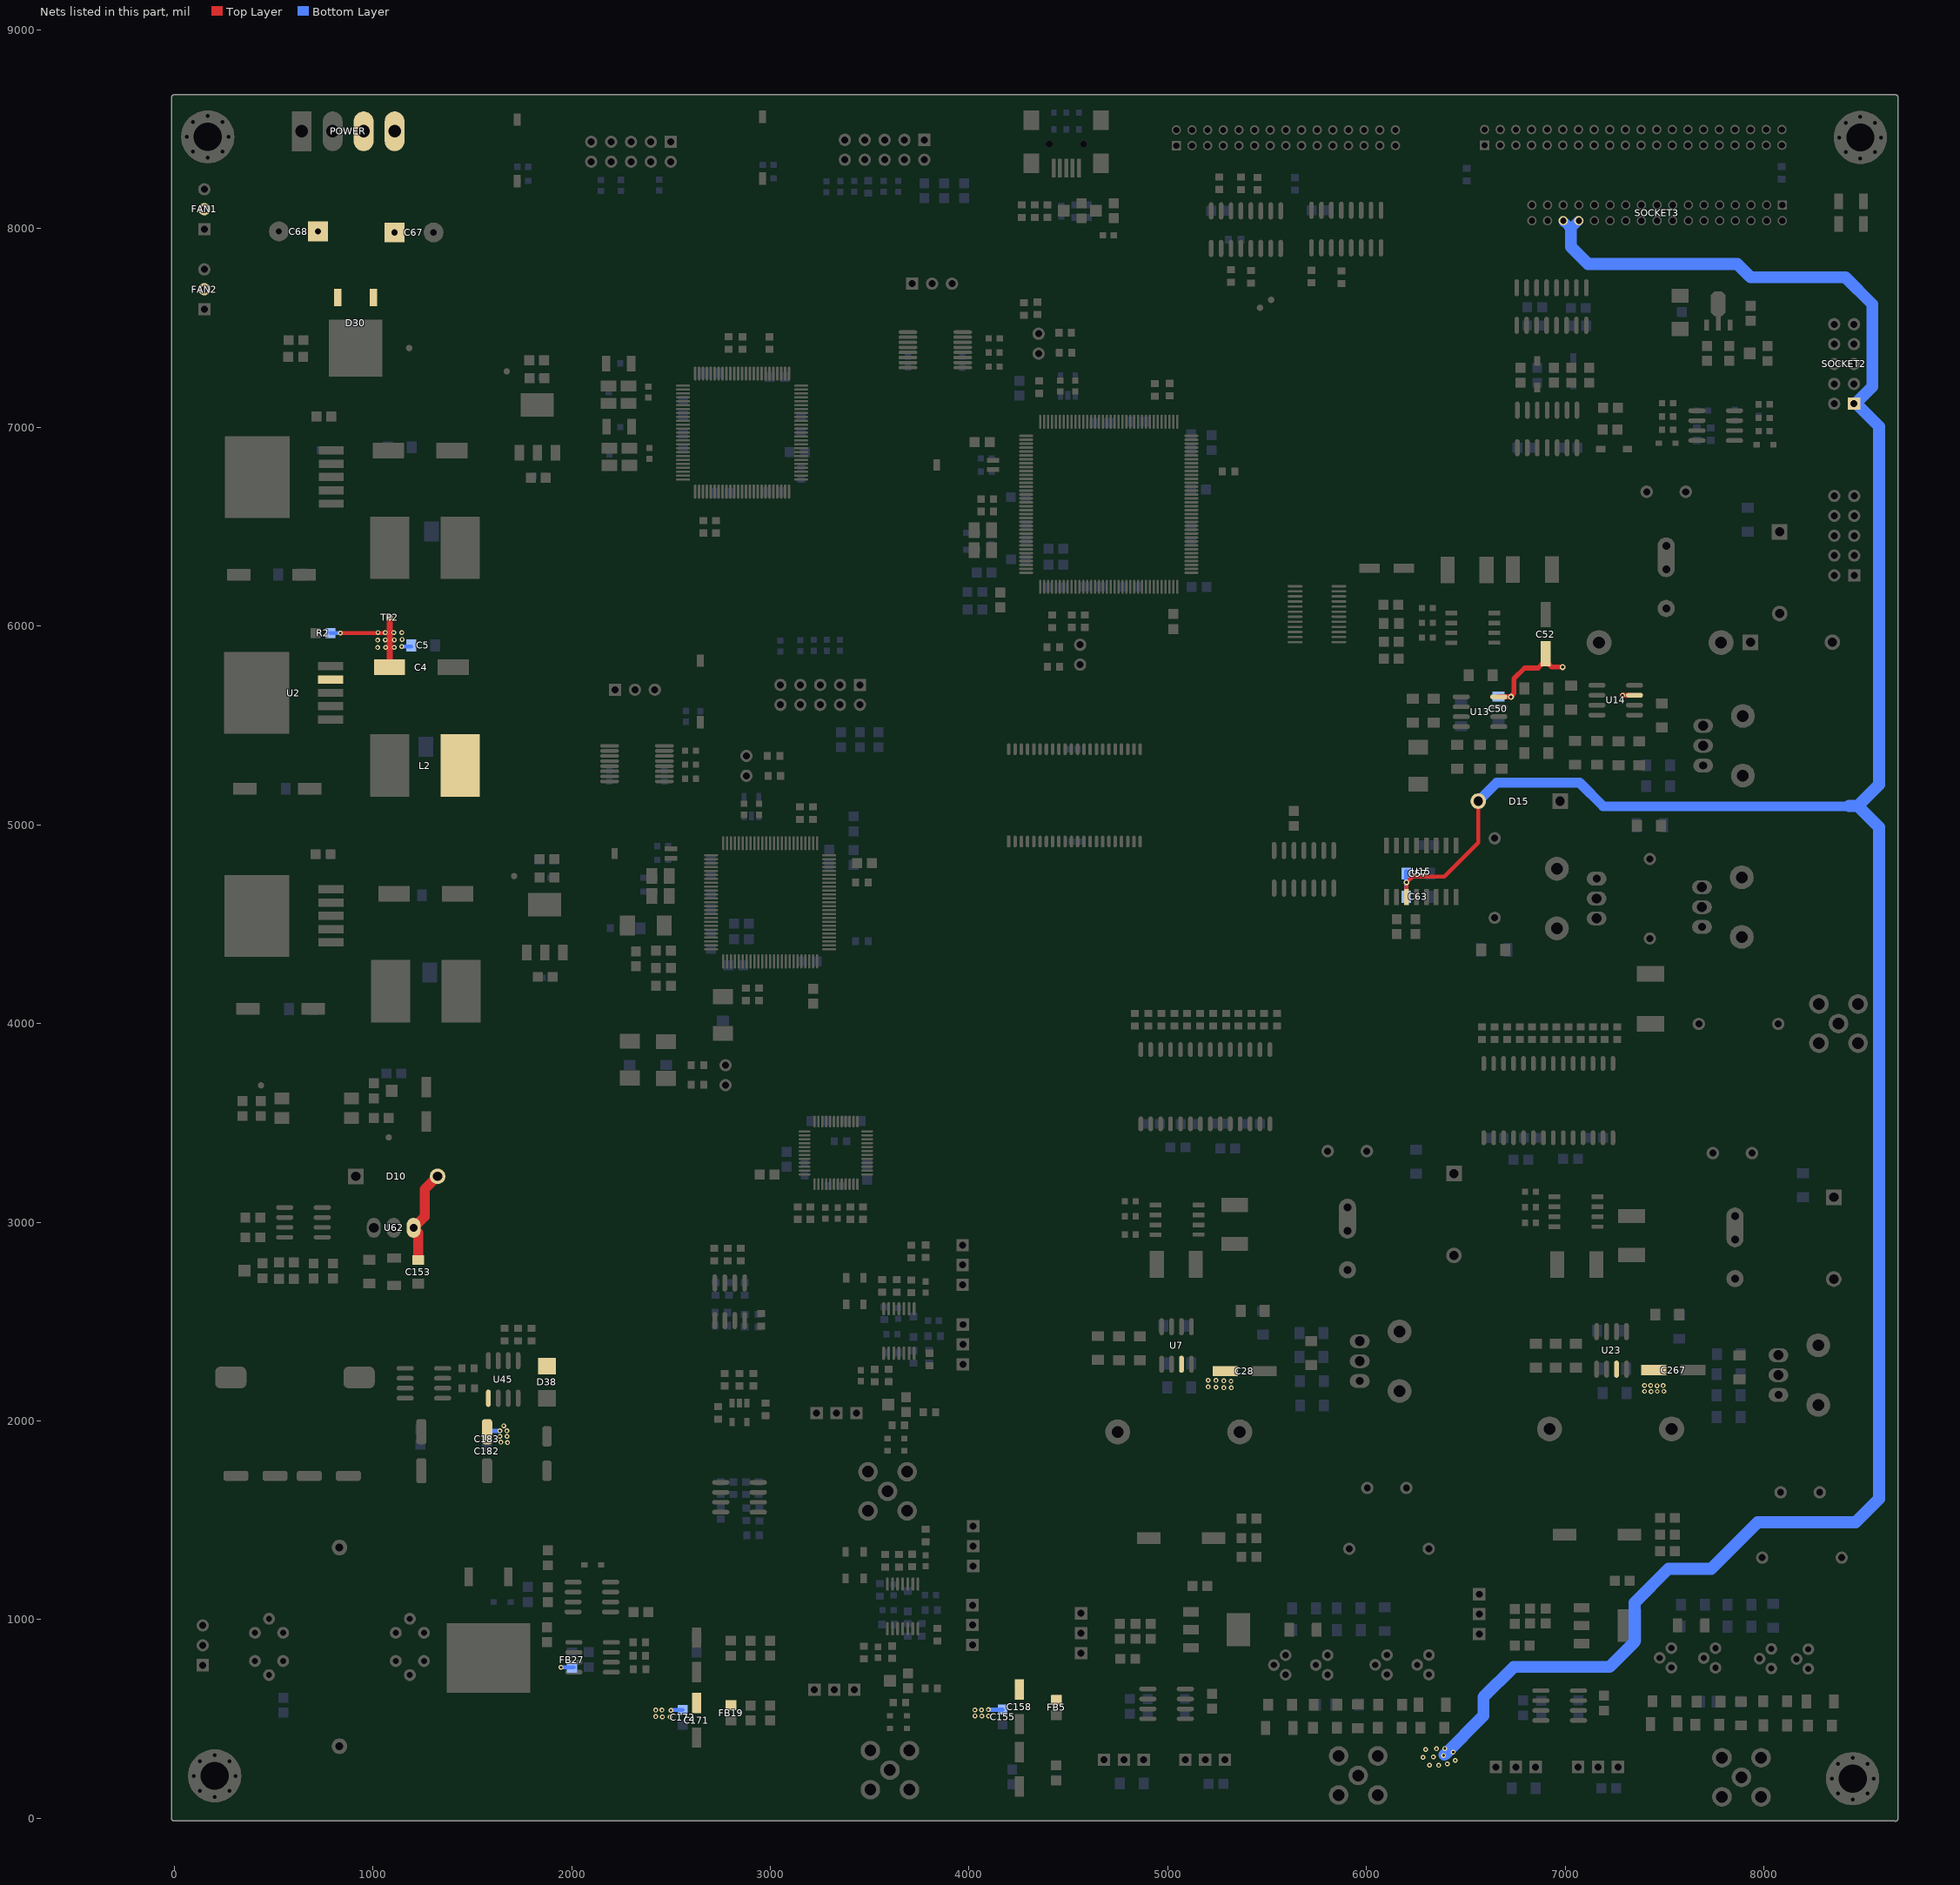
[diagram p0: the nets of this part, all layers, seen from the top]
# Altium PCB MISC82309.PcbDoc (part 4 of 14)
Units mil, origin at the board's own origin, x right, y up, seen from the top; angles counter-clockwise.
Board outline 8687.03 x 8687.86 mil, 4 copper layers (Top Layer, GND, POWER, Bottom Layer); 747 components, 583 nets, 2530 pads, 1834 vias.

## Footprints (in the part's own frame and the unit in brackets; to place one, negate y for a bottom-side part, rotate by r counter-clockwise, add the part's x,y. Pads: shape width x height; smd on the part's side, far side on the other; paste and mask are expansions set on the pad) (continued)
P-DSO-8 [mm]
  rect 1.5x0.6 smd: 1(0,0) 2(0,-1.27) 3(0,-2.54) 4(0,-3.81) 6(5.5,-2.54) 7(5.5,-1.27) 8(5.5,0)
  rect 1.5x0.5 smd: 5(5.5,-3.81)
  silkscreen extent 0.95,-4.51 4.55,0.7
PBS5022 [mm]
  rrect50% 4x2.79 smd: 1(-8.2,0) 2(8.2,0)
  silkscreen extent -9.27,-7.62 9.27,7.62, body extent -9.02,-7.37 9.02,7.37, height 7.51
PLS-2-2_54 [mil] "ZL201 SERIES 2.54 MM (0.100'') STRAIGHT PIN HEADER"
  round 62 hole 35: 1(0,0) 2(100,0)
  silkscreen extent -50,-50 150,50, body extent -50,-50 150,50, height 336
R0603 [mm]
  rect 0.8x0.8 smd: 1(-0.698,0) 2(0.698,0)
  silkscreen extent -1.46,-0.7 1.46,0.7, body extent -0.8,-0.4 0.8,0.4, height 0.4
R0805 [mil]
  rect 50x50 smd: 1(-37.5,0) 2(37.5,0)
  silkscreen extent -80,-38 80,38
R1206 [mil]
  rect 50x60 smd: 1(-60,0) 2(60,0)
  silkscreen extent -94,-41 94,41, body extent -63,-31 63,31, height 22
Radj [mil]
  rect 62x62 hole 35: 1(0,0) 2(100,0) 3(200,0)
  silkscreen extent -90,-110 290,103, body extent -88,-95 288,95, height 455
RES_0603 [mm]
  rect 0.9x1 smd: 1(-0.8,0) 2(0.8,0)
  silkscreen extent -1.45,-0.7 1.45,0.7, body extent -0.8,-0.4 0.8,0.41, height 0.4
RES_0805 [mil]
  rect 50x50 smd: 1(-37.5,0) 2(37.5,0)
  silkscreen extent -70,-32 70,32, body extent -39,-25 39,25, height 20
RES_2512 [mm]
  rect 2x3.5 smd: 1(-3.2,0) 2(3.2,0)
  silkscreen extent -4.45,-2.03 4.45,2.03, body extent -3.2,-1.6 3.2,1.6, height 0.6
RM8 [mil]
  round 60 hole 30: 1(-425.2,70.87) 2(-425.2,-70.87) 3(-354.33,141.73) 4(-354.33,-141.73) 5(-283.46,70.87) 6(-283.46,-70.87) 7(425.2,70.87) 8(425.2,-70.87) 9(354.33,141.73) 10(354.33,-141.73) 11(283.46,70.87) 12(283.46,-70.87)
  round 78.74 hole 39.37: M-1(0,500) M-2(0,-500)
  silkscreen extent -462,-329 462,329, body extent -466,-502 466,502, height 642
SB560 [mm]
  round 3.2 hole 1.524: 1(0,0) 2(15.6,0)
  silkscreen extent 2.54,-2.54 12.95,2.54, body extent -0.7,-2.79 16.2,2.85, height 5.82
SMB_V-RJ45#1 [mm] "Connector; SMB Straight"
  round 2.5 hole 1.5: 1(0,0) 2(-2.5,-2.5) 2(-2.5,2.5) 2(2.5,-2.5) 2(2.5,2.5)
  silkscreen extent -3.15,-3.15 3.15,3.15
SMB_V-RJ45#2 [mm] "Connector; SMB Straight"
  round 2.5 hole 1.5: 1(0,0) M-1(-2.5,2.5) M-2(2.5,2.5) M-3(2.5,-2.5) M-4(-2.5,-2.5)
  silkscreen extent -3.15,-3.15 3.15,3.15, body extent -3.5,-3.5 3.5,3.5, height 7.56
SMD0805-L [mm] "Molded Inductor, 2-Leads, Body 2.00x1.25mm, IPC Medium Density"
  rect 1.25x1.35 smd: 1(-0.975,0) 2(0.975,0)
  silkscreen extent -1.85,-0.94 1.85,0.94, body extent -1.1,-0.7 1.1,0.7, height 0.6
SMD1206-L [mm] "Chip Inductor, 2-Leads, Body 3.25x1.65mm, IPC Medium Density"
  rect 1.1x2 smd: 1(-1.6,0) 2(1.6,0)
  silkscreen extent -2.45,-1.26 2.45,1.24, body extent -1.75,-0.9 1.75,0.9, height 1.27
SMD1812-Fuse [mm] "Chip Fuse, 2-Leads, Body 4.55x3.24mm, IPC Medium Density"
  rect 1.8x3.4 smd: 1(-2.49,0) 2(2.49,0)
  silkscreen extent -3.68,-1.98 3.71,2.01, body extent -2.25,-1.6 2.25,1.6, height 0.38
SMD5032 [mm]
  rect 2x1.4 smd: 1(0,0) 2(2.54,0) 3(2.54,2.2) 4(0,2.2)
  silkscreen extent -1.22,-1.37 3.78,3.12
SO8 [mm] "SOIC, 8-Leads, Body 4.9x3.9mm, Pitch 1.27mm, IPC Medium Density"
  oval 2.2x0.6 smd: 1(-2.4,1.905) 2(-2.4,0.635) 3(-2.4,-0.635) 4(-2.4,-1.905) 5(2.4,-1.905) 6(2.4,-0.635) 7(2.4,0.635) 8(2.4,1.905)
  silkscreen extent -2.52,-2.5 0.9,2.88, body extent -3,-2.45 3,2.45, height 1.7
SO8_N [mm] "SOIC, 8-Leads, Body 4.9x3.9mm, Pitch 1.27mm, IPC Medium Density"
  oval 2.2x0.6 smd: 1(-2.4,1.905) 2(-2.4,0.635) 3(-2.4,-0.635) 4(-2.4,-1.905) 5(2.4,-1.905) 6(2.4,-0.635) 7(2.4,0.635) 8(2.4,1.905)
  silkscreen extent -2.53,-2.5 0.9,2.88, body extent -1.95,-2.45 1.95,2.45, height 1.75
SO14 [mm] "SOIC, 14-Leads, Body 8.7x3.9mm, Pitch 1.27mm, IPC Medium Density"
  oval 2.2x0.6 smd: 1(-2.4,3.81) 2(-2.4,2.54) 3(-2.4,1.27) 4(-2.4,0) 5(-2.4,-1.27) 6(-2.4,-2.54) 7(-2.4,-3.81) 8(2.4,-3.81) 9(2.4,-2.54) 10(2.4,-1.27) 11(2.4,0) 12(2.4,1.27) 13(2.4,2.54) 14(2.4,3.81)
  silkscreen extent -2.52,-4.4 0.9,4.78, body extent -3.07,-4.35 3.07,4.35, height 1.78
SO14_N [mm] "SOIC, 14-Leads, Body 8.7x3.9mm, Pitch 1.27mm, IPC Medium Density"
  oval 2.2x0.6 smd: 1(-2.4,3.81) 2(-2.4,2.54) 3(-2.4,1.27) 4(-2.4,0) 5(-2.4,-1.27) 6(-2.4,-2.54) 7(-2.4,-3.81) 8(2.4,-3.81) 9(2.4,-2.54) 10(2.4,-1.27) 11(2.4,0) 12(2.4,1.27) 13(2.4,2.54) 14(2.4,3.81)
  silkscreen extent -2.52,-4.4 0.9,4.79, body extent -1.95,-4.33 1.95,4.33, height 1.75
SO-8_N [mm] "SOIC, 8-Leads, Body 4.9x3.9mm, Pitch 1.27mm, IPC Medium Density"
  oval 2.2x0.6 smd: 1(-2.4,1.905) 2(-2.4,0.635) 3(-2.4,-0.635) 4(-2.4,-1.905) 5(2.4,-1.905) 6(2.4,-0.635) 7(2.4,0.635) 8(2.4,1.905)
  silkscreen extent -2.52,-2.5 0.9,2.88, body extent -2,-2.5 2,2.5, height 1.75
SOD323 [mm]
  rect 0.8x0.7 smd: 1(1.075,0) 2(-1.075,0)
  silkscreen extent -0.66,-0.68 0.66,0.68, body extent -1.35,-0.62 1.35,0.63, height 1.1
SOD-123 [mm] "SOD-123; 2 Leads; Body 2.7 x 1.6 mm, (LxW)"
  rect 1.2x0.8 smd: 1(-1.7,0) 2(1.7,0)
  silkscreen extent -0.89,-0.8 0.89,0.81, body extent -1.85,-0.8 1.85,0.8, height 1.25
SOD-323 [mm]
  rect 1x1 smd paste+0.02 mask+0.05: 1(0,0) 2(0,2.6)
  silkscreen extent -0.68,0.64 0.68,1.95, body extent -0.68,-0.26 0.68,2.86, height 1
SOIC-8 [mm] "SOIC, 8-Leads, Body 4.9x3.9mm, Pitch 1.27mm, IPC Medium Density"
  oval 2.2x0.6 smd: 1(-2.4,1.905) 2(-2.4,0.635) 3(-2.4,-0.635) 4(-2.4,-1.905) 5(2.4,-1.905) 6(2.4,-0.635) 7(2.4,0.635) 8(2.4,1.905)
  silkscreen extent -2.52,-2.5 0.9,2.88, body extent -3,-2.45 3,2.45, height 1.7
SOIC-16 [mil]
  rect 80x24 smd: 1(-130,175) 2(-130,125) 3(-130,75) 4(-130,25) 5(-130,-25) 6(-130,-75) 7(-130,-125) 8(-130,-175) 9(130,-175) 10(130,-125) 11(130,-75) 12(130,-25) 13(130,25) 14(130,75) 15(130,125) 16(130,175)
  silkscreen extent -209,-205 77,205
SOIC_4N [mm] "SOT143, 4-Leads, Body 4.77x9.80mm, Pitch 2.55mm, IPC Medium Density"
  rect 1.9x1.5 smd: 1(-4.45,1.275) 2(-4.45,-1.275) 3(4.45,-1.275) 4(4.45,1.275)
  silkscreen extent -4.58,-2.5 3.5,2.7, body extent -5,-2.47 5,2.48, height 3.83
SOIC_8N [mm] "SOIC, 8-Leads, Body 4.90x3.90mm, Pitch 1.27mm, IPC Medium Density"
  oval 2.2x0.6 smd: 1(-2.4,1.905) 2(-2.4,0.635) 3(-2.4,-0.635) 4(-2.4,-1.905) 5(2.4,-1.905) 6(2.4,-0.635) 7(2.4,0.635) 8(2.4,1.905)
  silkscreen extent -2.52,-2.5 0.9,2.88, body extent -3.1,-2.5 3.1,2.5, height 1.75
SOP127P1020X265-28N [mm] "SOP, 28-Leads, Body 17.90x7.50mm, Pitch 1.27mm, IPC Medium Density"
  oval 1.9x0.6 smd: 1(-4.75,8.255) 2(-4.75,6.985) 3(-4.75,5.715) 4(-4.75,4.445) 5(-4.75,3.175) 6(-4.75,1.905) 7(-4.75,0.635) 8(-4.75,-0.635) 9(-4.75,-1.905) 10(-4.75,-3.175) 11(-4.75,-4.445) 12(-4.75,-5.715) 13(-4.75,-6.985) 14(-4.75,-8.255) 15(4.75,-8.255) 16(4.75,-6.985) 17(4.75,-5.715) 18(4.75,-4.445) 19(4.75,-3.175) 20(4.75,-1.905) 21(4.75,-0.635) 22(4.75,0.635) 23(4.75,1.905) 24(4.75,3.175) 25(4.75,4.445) 26(4.75,5.715) 27(4.75,6.985) 28(4.75,8.255)
  silkscreen extent -4.87,-9.05 3.4,9.23, body extent -5.26,-9.04 5.41,9.04, height 2.39
SOT23-5_M [mm]
  rect 1.1x0.65 smd: 1(1.2,-0.95) 2(1.2,0) 3(1.2,0.95) 4(-1.2,0.95) 5(-1.2,-0.95)
  silkscreen extent -0.25,-1.95 1.32,1.5, body extent -0.87,-1.5 0.88,1.5, height 1.45
SOT89 [mm]
  rect 1.4x0.6 smd: 1(-1.673,1.5) 3(-1.673,-1.5)
  rect 1.8x0.6 smd: 2(-1.473,0)
  oct 3.2x1.9 smd: 2(1.027,0)
  silkscreen extent -1.95,-2.3 1.43,2.47, body extent -2.31,-2.31 1.94,2.29, height 1.6
SOT223 [mm]
  rect 2x1.2 smd: 1(0,0.014) 2(0,-2.286) 3(0,-4.586)
  rect 3x4.2 smd: 4(6.096,-2.272)
  silkscreen extent 1.27,-5.7 4.32,1.28, body extent -0.3,-5.51 6.7,0.99, height 1.7
SOT-23 [mil]
  rect 50x50 smd: 1(0,0) 2(0,-75)
  rect 60x60 smd: 3(90,-38)
  silkscreen extent 5,-95 95,20, body extent -5,-97 95,21, height 43
SOT-23-3 [mil]
  rect 50x50 smd: 1(-45,37.5) 2(-45,-37.5)
  rect 60x60 smd: 3(45,-0.5)
  silkscreen extent -40,-58 50,58, body extent -50,-60 50,59, height 43
SSOP16_M [mm] "SOP, 16-Leads, Body 6.2x5.3mm, Pitch 0.65mm, IPC Low Density"
  oval 2.4x0.45 smd: 1(-3.5,2.275) 2(-3.5,1.625) 3(-3.5,0.975) 4(-3.5,0.325) 5(-3.5,-0.325) 6(-3.5,-0.975) 7(-3.5,-1.625) 8(-3.5,-2.275) 9(3.5,-2.275) 10(3.5,-1.625) 11(3.5,-0.975) 12(3.5,-0.325) 13(3.5,0.325) 14(3.5,0.975) 15(3.5,1.625) 16(3.5,2.275)
  silkscreen extent -3.63,-3.25 1.9,3.25, body extent -3.81,-3.25 3.81,3.25, height 1.99
SW-6X3X2.5 [mil] "Switch, 6x3x2.5mm"
  rect 62.99x35 smd: 1(-155,0) 2(155,0)
  silkscreen extent -118,-69 118,69, body extent -157,-73 157,73, height 98
TO220 [mil]
  oval 100x70 hole 50: 1(0,100) 2(0,0)
  oval 100x70 hole 40: 3(0,-100)
  silkscreen extent -69,-200 131,200, body extent -55,-200 125,200, height 723
TO220V1 [mil]
  oval 100x70 hole 50: 1(0,100) 2(0,0)
  oval 100x70 hole 40: 3(0,-100)
  round 120 hole 59: M-1(200,150) M-2(200,-150)
  silkscreen extent -100,-383 321,384, body extent -55,-374 311,374, height 986
TO-92 [mm]
  round 1.5 hole 0.8: 1(0,-1.25) 2(-1.5,0) 3(0,1.25)
  silkscreen extent -2.66,-2.66 1.91,2.66, body extent -2.64,-2.67 1.52,2.65, height 8.33
TO-252AA [mm] "D-PAK, 3-Pads, Body 6.21x6.73mm (max), IPC Medium Density"
  rect 2.25x0.95 smd: 1(-4.45,2.28) 3(-4.45,-2.28)
  rect 7.3x6.8 smd: 4(2,0)
  silkscreen extent -4.57,-3.35 -2.05,3.43, body extent -4.7,-3.3 5,3.28, height 2.3
TPOINT [mil]
  round 32 smd: 1(0,0)
  silkscreen extent -25,-25 25,25
TQFP100_N [mm]
  oval 0.3x1.8 smd: 1(-6,-7.55) 2(-5.5,-7.55) 3(-5,-7.55) 4(-4.5,-7.55) 5(-4,-7.55) 6(-3.5,-7.55) 7(-3,-7.55) 8(-2.5,-7.55) 9(-2,-7.55) 10(-1.5,-7.55) 11(-1,-7.55) 12(-0.5,-7.55) 13(0,-7.55) 14(0.5,-7.55) 15(1,-7.55) 16(1.5,-7.55) 17(2,-7.55) 18(2.5,-7.55) 19(3,-7.55) 20(3.5,-7.55) 21(4,-7.55) 22(4.5,-7.55) 23(5,-7.55) 24(5.5,-7.55) 25(6,-7.55) 51(6,7.55) 52(5.5,7.55) 53(5,7.55) 54(4.5,7.55) 55(4,7.55) 56(3.5,7.55) 57(3,7.55) 58(2.5,7.55) 59(2,7.55) 60(1.5,7.55) 61(1,7.55) 62(0.5,7.55) 63(0,7.55) 64(-0.5,7.55) 65(-1,7.55) 66(-1.5,7.55) 67(-2,7.55) 68(-2.5,7.55) 69(-3,7.55) 70(-3.5,7.55) 71(-4,7.55) 72(-4.5,7.55) 73(-5,7.55) 74(-5.5,7.55) 75(-6,7.55)
  oval 1.8x0.3 smd: 26(7.55,-6) 27(7.55,-5.5) 28(7.55,-5) 29(7.55,-4.5) 30(7.55,-4) 31(7.55,-3.5) 32(7.55,-3) 33(7.55,-2.5) 34(7.55,-2) 35(7.55,-1.5) 36(7.55,-1) 37(7.55,-0.5) 38(7.55,0) 39(7.55,0.5) 40(7.55,1) 41(7.55,1.5) 42(7.55,2) 43(7.55,2.5) 44(7.55,3) 45(7.55,3.5) 46(7.55,4) 47(7.55,4.5) 48(7.55,5) 49(7.55,5.5) 50(7.55,6) 76(-7.55,6) 77(-7.55,5.5) 78(-7.55,5) 79(-7.55,4.5) 80(-7.55,4) 81(-7.55,3.5) 82(-7.55,3) 83(-7.55,2.5) 84(-7.55,2) 85(-7.55,1.5) 86(-7.55,1) 87(-7.55,0.5) 88(-7.55,0) 89(-7.55,-0.5) 90(-7.55,-1) 91(-7.55,-1.5) 92(-7.55,-2) 93(-7.55,-2.5) 94(-7.55,-3) 95(-7.55,-3.5) 96(-7.55,-4) 97(-7.55,-4.5) 98(-7.55,-5) 99(-7.55,-5.5) 100(-7.55,-6)
  silkscreen extent -6.82,-7.67 6.25,6.25, body extent -7,-7 7,7, height 1.6
TS5B_N [mm] "D2-PAK, 6-Leads, Body 8.6x10.2mm, Pitch 1.7mm, Lead Span 14.1mm, IPC Medium Density"
  rect 3.2x1.05 smd: 1(-6,3.4) 2(-6,1.7) 3(-6,0) 4(-6,-1.7) 5(-6,-3.4)
  rect 8.3x10.45 smd: 6(3.45,0)
  silkscreen extent -6.13,-5.2 -1.1,5.2, body extent -2.65,-5.2 6.24,5.2, height 4.65
TSOP44-IS61LV51216AL-10TLI [mm] "512K x 16 HIGH SPEED ASYNCHRONOUS  CMOS STATIC RAM WITH 3.3V SUPPLY"
  rect 1.5x0.45 smd: 1(0,0)
  oval 1.5x0.45 smd: 2(0,-0.8) 3(0,-1.6) 4(0,-2.4) 5(0,-3.2) 6(0,-4) 7(0,-4.8) 8(0,-5.6) 9(0,-6.4) 10(0,-7.2) 11(0,-8) 12(0,-8.8) 13(0,-9.6) 14(0,-10.4) 15(0,-11.2) 16(0,-12) 17(0,-12.8) 18(0,-13.6) 19(0,-14.4) 20(0,-15.2) 21(0,-16) 22(0,-16.8) 23(11.8,-16.8) 24(11.8,-16) 25(11.8,-15.2) 26(11.8,-14.4) 27(11.8,-13.6) 28(11.8,-12.8) 29(11.8,-12) 30(11.8,-11.2) 31(11.8,-10.4) 32(11.8,-9.6) 33(11.8,-8.8) 34(11.8,-8) 35(11.8,-7.2) 36(11.8,-6.4) 37(11.8,-5.6) 38(11.8,-4.8) 39(11.8,-4) 40(11.8,-3.2) 41(11.8,-2.4) 42(11.8,-1.6) 43(11.8,-0.8) 44(11.8,0)
  silkscreen extent 1.58,-17.2 10.3,0.4, body extent 0.03,-17.54 11.79,0.67, height 1.3
TSSOP-24 [mm]
  oval 1.9x0.3 smd: 1(-2.8,3.575) 2(-2.8,2.925) 3(-2.8,2.275) 4(-2.8,1.625) 5(-2.8,0.975) 6(-2.8,0.325) 7(-2.8,-0.325) 8(-2.8,-0.975) 9(-2.8,-1.625) 10(-2.8,-2.275) 11(-2.8,-2.925) 12(-2.8,-3.575) 13(2.8,-3.575) 14(2.8,-2.925) 15(2.8,-2.275) 16(2.8,-1.625) 17(2.8,-0.975) 18(2.8,-0.325) 19(2.8,0.325) 20(2.8,0.975) 21(2.8,1.625) 22(2.8,2.275) 23(2.8,2.925) 24(2.8,3.575)
  silkscreen extent -1.6,-4 1.6,4
U5+1_N [mm] "SOT23, 5-Leads, Body 2.9x1.6mm, Pitch 0.95mm, Lead Span 2.8mm, IPC Medium Density"
  rect 1.1x0.65 smd: 1(-1.2,0.95) 2(-1.2,0) 3(-1.2,-0.95) 4(1.2,-0.95) 5(1.2,0.95)
  silkscreen extent -1.32,-1.5 0.25,1.95, body extent -0.87,-1.5 0.87,1.5, height 1.45
VH-3_96-4 [mm]
  rect 2.54x5.08 hole 1.6: 1(0,0)
  oval 2.54x5.08 hole 1.6: 2(3.96,0) 3(7.92,0) 4(11.88,0)
  silkscreen extent -1.98,-4.8 13.86,3.7, body extent -1.95,-4.8 13.83,3.7, height 10.73
Y_XTAL_T7 [mm]
  rect 0.6x1.6 smd: 1(1.235,0.254) 4(0.035,0.254)
  rect 0x0 smd: 2(0.635,6.858)
  rect 1.4x0.8 smd: 3(0.635,7.454)
  silkscreen extent -0.17,0.25 1.44,7.25, body extent -0.24,-0.38 1.51,7.56, height 1.6

## Part data
C1 C2 C6 C7 C8 C14 C16 C18 C19 C20 C34 C39 C40 C41 C65 C66 C74 C75 C79 C80 C81 C84 C85 C86 C87 C88 C89 C98 C99 C123 C124 C125 C126 C127 C128 C129 C130 C131 C132 C133 C134 C141 C142 C143 C146 C147 C148 C172 C173 C175 C176 C193 C195 C196 C197 C198 C199 C200 C201 C202 C242 C243 C244 C245 C246 C247 C248 C249 C250 C251 C252 C253 C254 C255 C449: library part CAP_1206, "Capacitor"
C3 C4 C9 C10 C11 C12: library part "CAP POL"
C5 C13 C15 C42 C155 C156 C280 C281: library part CAP_0.1uF
C17 C64 C158 C159 C171 C174: library part CAP_POLAR_1, "Polar Capacitor"
C23 C47 C265: library part CAP_47pF, "Capacitor 47pF"
C24 C49 C270: library part CAP_10nF, "Capacitor 10nF"
C25 C48 C271: library part CAP_2.2nF, "Capacitor 2.2nF"
C27 C51 C263: library part CAP_470pF, "Capacitor 470pF"
C28 C52 C267: library part CAP_POLAR_22uF_35V, "Polar Capacitor 22uF 35V"
C29 C54 C266: library part CAP_POLAR_2.2uF_450V, "Polar Capacitor 222uF 450V"
C30 C31 C32 C33 C56 C63 C153 C157 C277 C282 C283 C284 C285 C317 C318: library part CAP_0.1uF, "Capacitor 0.1uF"
C35 C36 C37 C38 C70 C71 C72 C73 C82 C83 C151 C154 C162 C183 C184 C214 C215 C220 C221 C231 C233 C256 C257 C373 C374: library part CAP_0805, "Capacitor"
C45: library part CAP_0.22uF, "Capacitor 0.22uF"
C50 C53 C69 C278: library part CAP_0.47uF, "Capacitor 0.47uF"
C55 C188 C279: library part CAP_CBB_0.33uF_400V, "CBB Capacitor 0.33uF 400V"
C57: library part CAP_AVX_4.7uF_16V, "AVX Capacitor 4.7uFF 16V"
C58: library part CAP_CBB_0.1uF_400V, "CBB Capacitor0.1uF 400V"
C62: library part CAP_CBB_22nF_630V, "CBB Capacitor 22nF 630V"
C67 C68: library part CAP_EL, "Capacitor"
C78: library part CAP_0.1uF, "Capacitor 0.33uF"
C90 C91 C92 C93 C94 C177 C178 C179 C180 C181: library part CAP_0402, "Capacitor"
C163 C164 C363 C364: library part Cap, "Capacitor"
C165 C166 C167 C168 C169 C170 C210 C226 C232 C240 C241 C288 C289 C290 C291 C292 C293 C311 C330 C370 C411 C412 C413 C420 C421 C422 C423 C424 C501 C502 C599: library part CAP_0603, "Capacitor"
C182 C227 C228 C229 C230: library part CAP_ALU, "Capacitor"
C187 C276: library part CAP_0.22nF, "Capacitor 0.22nF"
C506 C507: "Capacitor (Semiconductor SIM Model)"
CH-DET_A CH-DET_B CHARGE-OUT_A CHARGE-OUT_B MOD-OUT: "SMB Straight Connector"
CPLD-JTAG D-JTAG P-JTAG SOCKET1 SOCKET2: library part HEAD2X5-2_54
D10: library part UF400X
D23 D28 D29 D34: "1SMA4728A 1W 3.3V SMA DO-214AC"
D24 D52 D54: library part BZT52C4V7
D27 D48: library part Diode-SMD
D40: library part UF4007
D55: library part 1N4001/M1
ESD23 ESD24 ESD25: library part DIODE_TVS_BI-DIR, "TVS,BIDIRECTION,5V,RENESAS PROJECT"
FB1 FB3 FB4 FB5 FB6 FB18 FB19 FB20 FB25 FB26 FB27: library part FB, "Res"
FUSE1 FUSE2 FUSE12 FUSE13 FUSE14 FUSE15: library part FUSE, "Res"
L2 L3 L4 L11 L13 L14 L21: library part Inductor
L5 L6 L15: library part "Toroidal Inductor"
L16 L111: library part "Power Inductance"
P21: library part USB_Slave
PCB_MH1 PCB_MH2 PCB_MH3 PCB_MH4: library part MOUNTING_HOLE_3MM, "Mounting Hole, M3 Screw, Plated, Square Pad"
Q1: library part Triode-NPN
Q3: "PNP General  Purpose Transistors"
Q4 Q9 Q16 Q22 V3 V4: "HEXFET N-Channel Power MOSFET"
Q7 Q19 Q20: library part NPN
Q8: library part SI2301, "MOSFET"
Q10: "P-Channel 30V (D-S) Rated  MOSFET"
Q26: library part MOSFET-N, "N-Channel MOSFET"
R1 R2 R3 R4 R5 R6 R7 R8 R9 R11 R12 R13 R15 R16 R155 R156 R165 R166 R168 R212 R215 R216 R217 R220 R222 R225 R235 R269 R276 R277 R283 R284 R293 R386 R399 R491 R493 R495 R496: library part Res_0805, "Res"
R17 R221: library part Res_1K8, "Resistance 1.8K"
R18 R163 R227 R305: library part Res_150K, "Resistance 150K"
R19 R236: library part Res_68K, "Resistance 68K"
R22 R33 R47 R290 R314 R316: library part Res_50R, "Resistance 50R"
R23 R98: library part Res_22R, "Resistance 22R"
R25 R43 R82 R159 R297: library part Res_1K, "Resistance 1K"
R26 R160: library part Res_8K2, "Resistance 8.2K"
R27 R44 R291 R315: library part Res_470R, "Resistance 470R"
R28 R157: library part Res_4R7, "Resistance 4.7R"
R29 R158: library part Res_2R2, "Resistance 2R2"
R30 R34 R317 R318: library part Res_20R, "Resistance 20R"
R31 R164 R306 R320: library part Res_2K, "Resistance 2K"
R32 R89 R152 R203 R303 R304 R321: library part Res_100R, "Resistance 100R"
R35 R36 R57 R61 R62 R64 R65 R95 R96 R101 R102 R103 R104 R150 R186 R187 R188 R189 R190 R191 R192 R193 R194 R195 R196 R197 R198 R199 R200 R213 R214 R226 R270 R271 R272 R273 R274 R275 R285 R286 R287 R288 R322 R323 R324 R325 R326 R327 R328 R329 R330 R331 R332 R333 R334 R336 R339 R345 R346 R347 R348 R349 R358 R378 R379 R391 R392 R404 R405 R406 R407 R408 R409 R410 R411 R412 R413 R414 R415 R416 R417 R418 R419 R455 R478 R479 R508 R509 R511 R513 R514 R515 R516 R517 R518 R519 R521 R522 R523 R524 R525 R526 R527 R528 R529 R530 R531 R532 R533 R534 R535 R536 R537 R538 R539 R540 R541 R542 R543 R544 R545 R546 R547 R548 R549 R550 R555 R556 R558 R564 R565 R567 R569 R578 R598 R599: library part Res_0603, "Res"
R38 R39 R71 R74 R313 R319: library part Res_1M, "Resistance 1M"
R40 R41 R298 R299: library part Res_1K5, "Resistance 1.5K"
R42 R201 R300 R301: library part Res_390R, "Resistance 390R"
R45 R46 R295 R296: library part Res_2K7, "Resistance 2.7K"
R48 R292: library part Res_3K3, "Resistance 3.3K"
R58 R59 R106 R108 R109 R110 R206 R207 R232 R234 R294 R587 R588 R589 R590 R591 R592 R593 R594 R595 R596: library part Res
R63 R66 R67 R68 R72 R91 R100 R111 R112 R113 R114 R149 R151 R172 R173 R174 R175 R204 R205 R208 R209 R312 R343 R344 R372 R373 R374 R375: library part Res2, "Resistor"
R70 R73 R79 R80: library part Res_20K
R75: library part Res_8K2
R76 R78: library part Res_22K
R77: library part Res_150K
R81: library part Res_22R
R84: library part Res_2R2
R85: library part Res_1R
R87 R92: library part Res_220R, "Resistance 220R"
R153 R154 R161 R162 R307 R308 R309 R310: library part Res_12K, "Resistance 12K"
R202 R302: library part Res_2K2, "Resistance 2.2K"
Radj1 Radj3 Radj6 Radj10 Radj11 Radj12: library part Radj
Radj2 Radj9: library part Res_Adj_10K
Radj4 Radj8: library part Res_Adj_2K
Radj5 Radj7: library part Res_Adj_5K
T1: "Three-winding Transformer (Non-Ideal)"
TC2 TC3: library part CAP_POLAR_220uF_25V, "Polar Capacitor 220uF 25V"
TP1 TP2 TP3 TP4 TP5 TP6 TP7 TP8: "Test Point"
U1 U6: library part REG1117-3, "1A Low Dropout Positive Regulator Fixed"
U2 U3 U4: "SIMPLE SWITCHER?Power Converter 150 KHz 3A Step-Down Voltage Regulator, 5-pin TO-263"
U7 U14 U23: library part UC3842N, "Current Mode PWM Controller"
U10: "ARM Cortex-M4 32-bit MCU+FPU, 210 DMIPS, 512 kB Flash, 192 kB Internal RAM, 114 I/Os, 144-pin LQFP, -40 to 85 degC, Tray"
U12 U57 U58: library part I742RI
U13: "General-Purpose J-FET Dual Operational Amplifier"
U15: library part IR2110, "High and Low Side Driver"
U16: "MAX II 1.8V CPLD, 80 IOs, 240 Logic Elements, 100-Pin Plastic TQFP, Commercial Temperature, Speed Grade 5, Pb-Free"
U17: "ARM Cortex-M4 32-bit MCU+FPU, 210 DMIPS, 1024 kB Flash, 192 kB Internal RAM, 82 I/Os, 100-pin LQFP, -40 to 85 degC, Tray"
U18 U38: "I²C/SMBus Silicon Serial Number, 5-pin SOT23, -40?to + 85?C, Pb-Free, Tape and Reel"
U21 U22 U31: "Quad EIA-422/423 Line Receiver"
U24 U37: library part MAX3232
U32 U49: "Hex Schmitt Inverter"
U33 U40: "Dual Low-Power Operational Amplifier"
U36 U51: "Single-Supply 3 to 44 V Operational Amplifier"
U47: "High Speed Dual MOSFET Driver"
U48 U107: "EXCALIBUR HIGH-SPEED JFET-INPUT  OPERATIONAL AMPLIFIERS"
U52: "Octal Bus Transceiver and 3.3-V to 5-V Shifter with 3-State Outputs"
U61 U63: library part AD8138
U62: "3-Terminal Positive Fixed Voltage Regulator"
U64: library part AD9288
V1: library part "Zener diode 3V3"
V6 V102: "NPN High Voltage Transistor"
V7 V103: "PNP High Voltage Transistor"
V8 V101: "NPN high-voltage transistors"
V10 V11 V12 V13: library part BZT52C3V3
X1 X3: library part SOC_24M
X2 X7: library part CRYSTAL-SMD4
X5 X8: library part CRYSTAL-SMD4A

## Via types
v1: diameter 24, hole 12, Top Layer to Bottom Layer, 1799 vias
v2: diameter 30, hole 15, Top Layer to Bottom Layer, 26 vias
v3: diameter 40, hole 20, Top Layer to Bottom Layer, 9 vias

## Nets (pads, with @x,y where several pads share a name; then routed paths per layer and width w, separated by ;. In a path a pad name is that pad's centre, name@x,y a point inside that pad or via, vN(x,y) a via of type N, cw(c..) or ccw(c..) an arc to the next point about the centre after c; other vN are vias at no path point)
24V_IN: C67.1 C68.1 D30.1 D30.3 FAN1.2 FAN2.2 POWER.3 POWER.4
+12V: C4.1 C5.1 C57.1 C63.2 C155.1 C158.1 C171.1 C172.2 C182.2 C183.2 D15.1 D38.1 FB5.1 FB19.1 FB27.2 L2.2 R2.1 SOCKET2.1 SOCKET3.28 SOCKET3.30 TP2.1 U2.4 U15.3 U45.5 | length 14591.4
  Top Layer w20: v1(837,5965) 1080,5965 ; U15.3@6201,4636 v2(6201,4710) ; v2@6202,4711 6231,4740 6392,4740 6562.09,4910.09 D15.1@6562.09,5119
  Top Layer w30: C4.1@1082,5798 1085,5801 TP2.1@1085,6044
  Bottom Layer w20: R2.1@787.5,5965 v1(837,5965) ; v1@1146,5897 1192,5897 C5.1@1193,5898 ; C183.2@1575,1946.5 1578.5,1950 v1@1638,1950 ; v1(1947,760) 1947.39,759.61 FB27.2@2012,759.61 ; v1@2503,545 2558.5,545 C172.2@2559,545.5 ; v1@4101,547 4168.5,547 C155.1@4169,547.5 ; C63.2@6200,4645 C57.1@6200,4755 C57.1@6200,4767
  Bottom Layer w50: D15.1@6562.09,5119 6655.09,5212 7072,5212 7191,5093 8427,5093 ; SOCKET3.30@6994,8034 7028,8000 7028,8001 SOCKET3.28@7066,8039
  Bottom Layer w60: v1@6392,320 6588,516 6588,610 6740,762 7222,762 7349,889 7349,1086 7519,1256 7735,1256 7969,1490 8461,1490 8579,1608 8579,4988 8472,5095 ; 7028,8000 7028,7909 7115,7822 7866,7822 7932,7756 8409,7756 8545,7620 8545,7205 8462,7122 8579,7005 8579,5202 8472,5095 ; 8427,5095 8472,5095
  other v1: 6363,267 6317,268 6406,274 6446,292 6284,307 6336,309 6388,317 6436,333 6298,347 6352,350 6394,352 2496,510 2457,511 2424,512 4064,515 4098,515 4030,516 2500,544 2424,545 2455,545 4029,546 4063,546 4097,547 1678,1891 1644,1893 1639,1922 1675,1922 1639,1950 1674,1950 1659,1976 1024,5892 1064,5893 1107,5893 1145,5897 1024,5929 1063,5931 1108,5931 1148,5933 1063,5967 1105,5967 1146,5967 1026,5968
+18V: C28.1 C50.1 C52.1 C153.1 C267.1 D10.1 U7.7 U13.8 U14.7 U23.7 U62.3 | length 1079.5
  Top Layer w25: U13.8@6665.49,5644 6724,5644 6742,5662 6742,5736 6795,5789 6863,5789 C52.1@6891,5817 ; C52.1@6901,5861 6901,5824 6931,5794 v2(6987,5794) ; v1(7288,5652) U14.7@7348.49,5652
  Top Layer w50: C153.1@1229,2810 1229,2948 U62.3@1205,2972 1261.5,3028.5 1261.5,3166.59 D10.1@1325.91,3231
  Bottom Layer w25: C50.1@6664,5645 v2@6726,5645
  other v1: 7432,2148 7399,2149 7463,2149 7496,2149 5282,2167 5320,2167 5242,2170 5203,2171 7462,2177 7493,2178 7399,2179 7430,2179 5318,2201 5282,2202 5242,2204 5203,2205
  other v2: 6727,5644